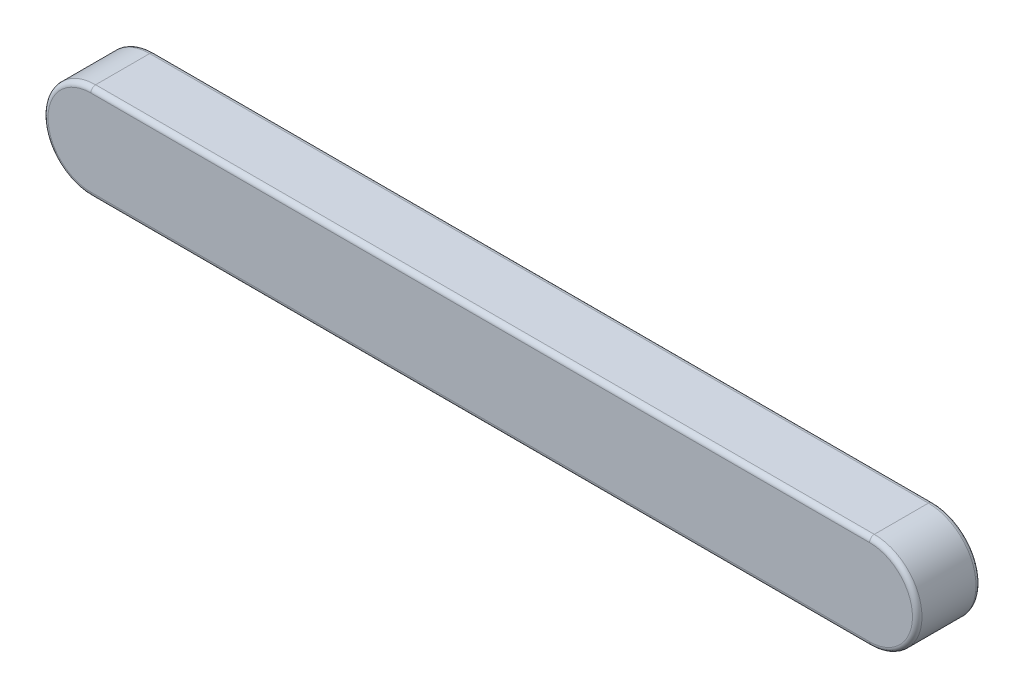
from build123d import *

# Parameters (mm, degrees)
EXTRUDE_523_DEPTH = 8
FILLET_1_R        = 0.6


with BuildPart() as part:
    # 草图1 → Extrude 523 (new body)
    with BuildSketch(Plane.XY):
        with BuildLine():
            Line((-49, 6), (49, 6))
            ThreePointArc((49, 6), (55, 0), (49, -6))
            Line((49, -6), (-49, -6))
            ThreePointArc((-49, -6), (-55, 0), (-49, 6))
        make_face()
    extrude(amount=EXTRUDE_523_DEPTH)

    # 圆角1
    fillet_1_edges = [part.edges().sort_by_distance(p)[0] for p in [
        (55, 0, 8),
        (0, 6, 8),
        (-55, 0, 8),
        (0, 6, 0),
        (55, 0, 0),
        (0, -6, 0),
        (-55, 0, 0),
        (0, -6, 8),
    ]]
    fillet(fillet_1_edges, radius=FILLET_1_R)


solid = part.part
